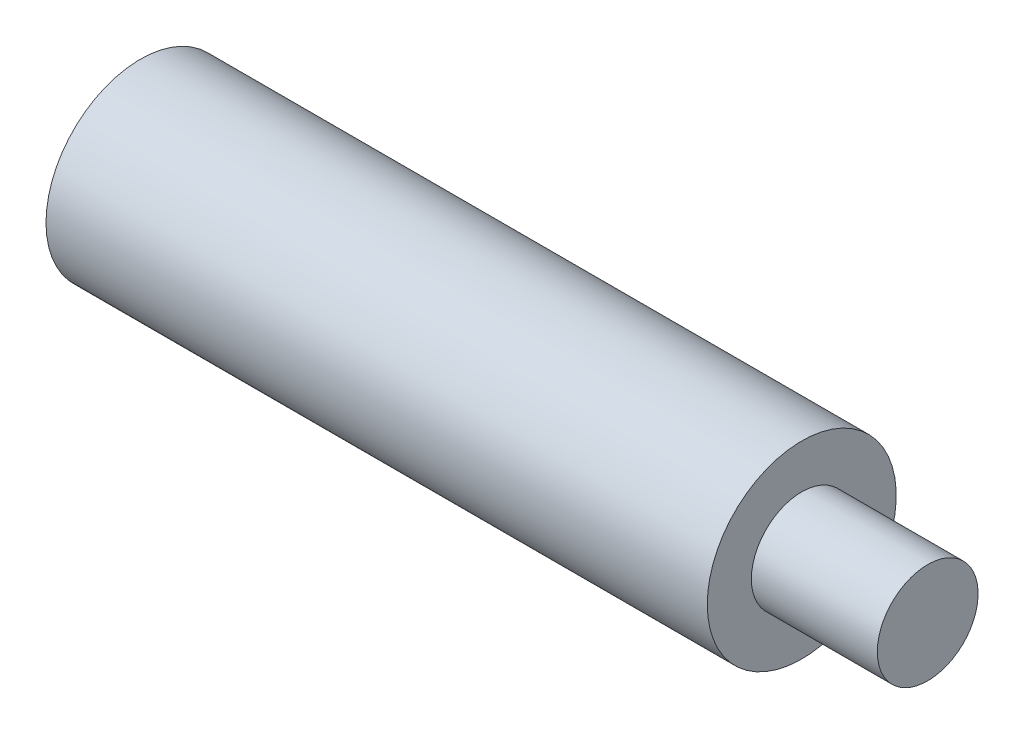
from build123d import *


with BuildPart() as part:
    # Sketch1 → Revolve1 (revolve)
    with BuildSketch(Plane.XY, mode=Mode.PRIVATE) as revolve1_sk:
        Polygon((0, 0), (0, 15), (105, 15), (105, 8), (125, 8), (125, 0), align=None)
    revolve(revolve1_sk.sketch.rotate(Axis((0, 0, 0), (1, 0, 0)), 90), axis=Axis((0, 0, 0), (1, 0, 0)))


solid = part.part
